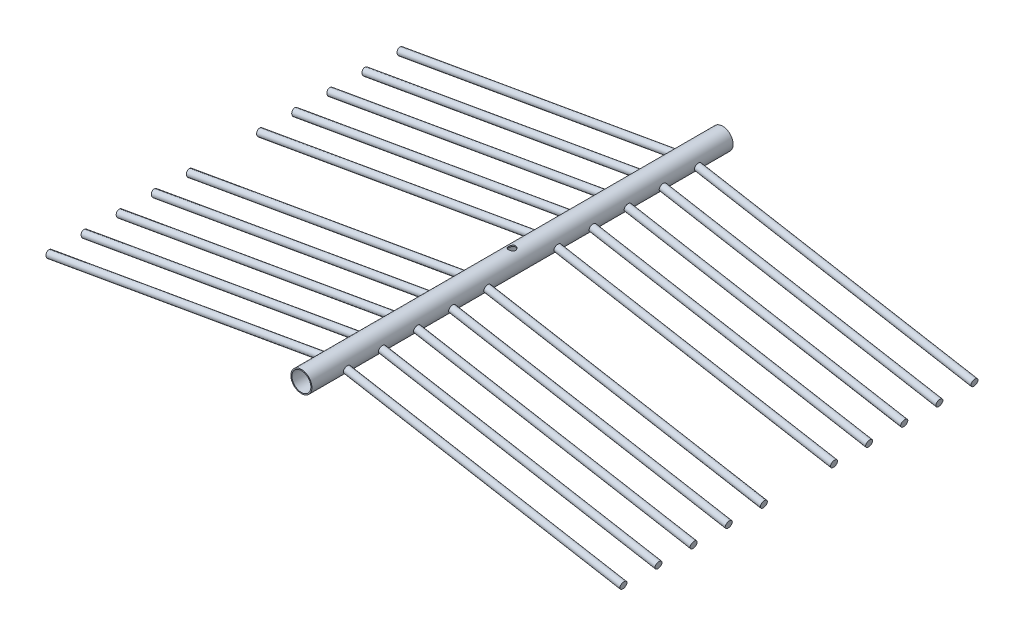
SolidWorks part; units mm, degrees
ref_plane "Front Plane" through (0, 0, 0) normal (0, 0, 1) x (1, 0, 0)
ref_plane "Top Plane" through (0, 0, 0) normal (0, 1, 0) x (1, 0, 0)
ref_plane "Right Plane" through (0, 0, 0) normal (1, 0, 0) x (0, 0, -1)
other "Configuration Table"
sketch "Sketch1" plane through (0, 0, 0) normal (0, 0, 1) x (1, 0, 0)
  circle A0 centre (0, 0) radius 15
  dimension "D1" = 30
extrude "Boss-Extrude1" add sketch "Sketch1" along normal blind 600
sketch "Sketch3" plane through (0, 0, 0) normal (1, 0, 0) x (0, 0, -1)
  line L0 (-300, 0) -> (0, 0) construction
  line L1 (-300, 15) -> (-300, -15) construction
  line L2 (0, 15) -> (-600, 15) construction
  line L3 (-600, -15) -> (0, -15) construction
  line L4 (-300, 0) -> (-600, 0) construction
  line L5 (-600, 15) -> (-600, -15) construction
  circle A0 centre (-550, 0) radius 5
  circle A1 centre (-500, 0) radius 5
  circle A2 centre (-450, 0) radius 5
  circle A3 centre (-400, 0) radius 5
  circle A4 centre (-350, 0) radius 5
  circle A5 centre (-250, 0) radius 5
  circle A6 centre (-200, 0) radius 5
  circle A7 centre (-150, 0) radius 5
  circle A8 centre (-100, 0) radius 5
  circle A9 centre (-50, 0) radius 5
  dimension "D1" = 10
  dimension "D2" = 10
  dimension "D3" = 10
  dimension "D4" = 10
  dimension "D5" = 10
  dimension "D6" = 50
  dimension "D7" = 50
  dimension "D8" = 50
  dimension "D9" = 50
  dimension "D10" = 50
ref_plane "Plane3" through (-14.7721, -2.6047, 0) normal (-0.9848, -0.1736, 0) x (0, 0, -1)
ref_plane "Plane4" through (14.7721, -2.6047, 0) normal (0.9848, -0.1736, 0) x (0, 0, -1)
sketch "Sketch5" plane through (-14.7721, -2.6047, 0) normal (-0.9848, -0.1736, 0) x (0, 0, -1)
  line L0 (-300, -89.4116) -> (-300, 91.219) construction
  line L1 (-600, -15) -> (0, -15) construction
  line L2 (-600, 0) -> (0, 0) construction
  line L3 (-600, 15) -> (-600, -15) construction
  circle A0 centre (-350, 0) radius 5
  circle A1 centre (-400, 0) radius 5
  circle A2 centre (-450, 0) radius 5
  circle A3 centre (-500, 0) radius 5
  circle A4 centre (-550, 0) radius 5
  circle A5 centre (-250, 0) radius 5
  circle A6 centre (-200, 0) radius 5
  circle A7 centre (-150, 0) radius 5
  circle A8 centre (-100, 0) radius 5
  circle A9 centre (-50, 0) radius 5
  point P14 (-300, 0)
  dimension "D4" = 10
  dimension "D2" = 50
  dimension "D3" = 15
  dimension "D8" = 50
  dimension "D9" = 50
  dimension "D10" = 50
  dimension "D11" = 50
extrude "Boss-Extrude3" add sketch "Sketch5" along normal blind 400 separate body contours A4 | A3 | A2 | A1 | A0 | A6 | A7 | A5 | A8 | A9
sketch "Sketch6" plane through (14.7721, -2.6047, 0) normal (0.9848, -0.1736, 0) x (0, 0, -1)
  line L2 (-300, 90.8706) -> (-300, -101.9168) construction
  circle A0 centre (-550, 0) radius 5
  circle A1 centre (-500, 0) radius 5
  circle A2 centre (-450, 0) radius 5
  circle A3 centre (-400, 0) radius 5
  circle A4 centre (-350, 0) radius 5
  circle A5 centre (-250, 0) radius 5
  circle A6 centre (-200, 0) radius 5
  circle A7 centre (-150, 0) radius 5
  circle A8 centre (-100, 0) radius 5
  circle A9 centre (-50, 0) radius 5
  point P13 (-300, -5.5231)
  dimension "D1" = 10
  dimension "D2" = 50
  dimension "D3" = 50
  dimension "D4" = 50
  dimension "D5" = 50
  dimension "D6" = 50
extrude "Boss-Extrude4" add sketch "Sketch6" along normal blind 400 separate body contours A0 | A1 | A2 | A3 | A4 | A5 | A6 | A8 | A7 | A9
sketch "Sketch7" plane through (0, 0, 0) normal (0, 1, 0) x (1, 0, 0)
  line L0 (-15, -300) -> (15, -300)
  line L1 (-15, 0) -> (-15, -600) construction
  line L2 (15, -600) -> (15, 0) construction
  line L3 (0, 0) -> (0, -600) construction
  line L4 (0, -300) -> (0, -600) construction
  circle A0 centre (0, -300) radius 5
  dimension "D1" = 10
extrude "Cut-Extrude1" cut sketch "Sketch7" along normal through all contours A0
sketch "Sketch8" plane through (0, 0, 600) normal (0, 0, 1) x (1, 0, 0)
  circle A0 centre (0, 0) radius 13.5
  dimension "D1" = 27
extrude "Cut-Extrude2" cut sketch "Sketch8" against normal through all
